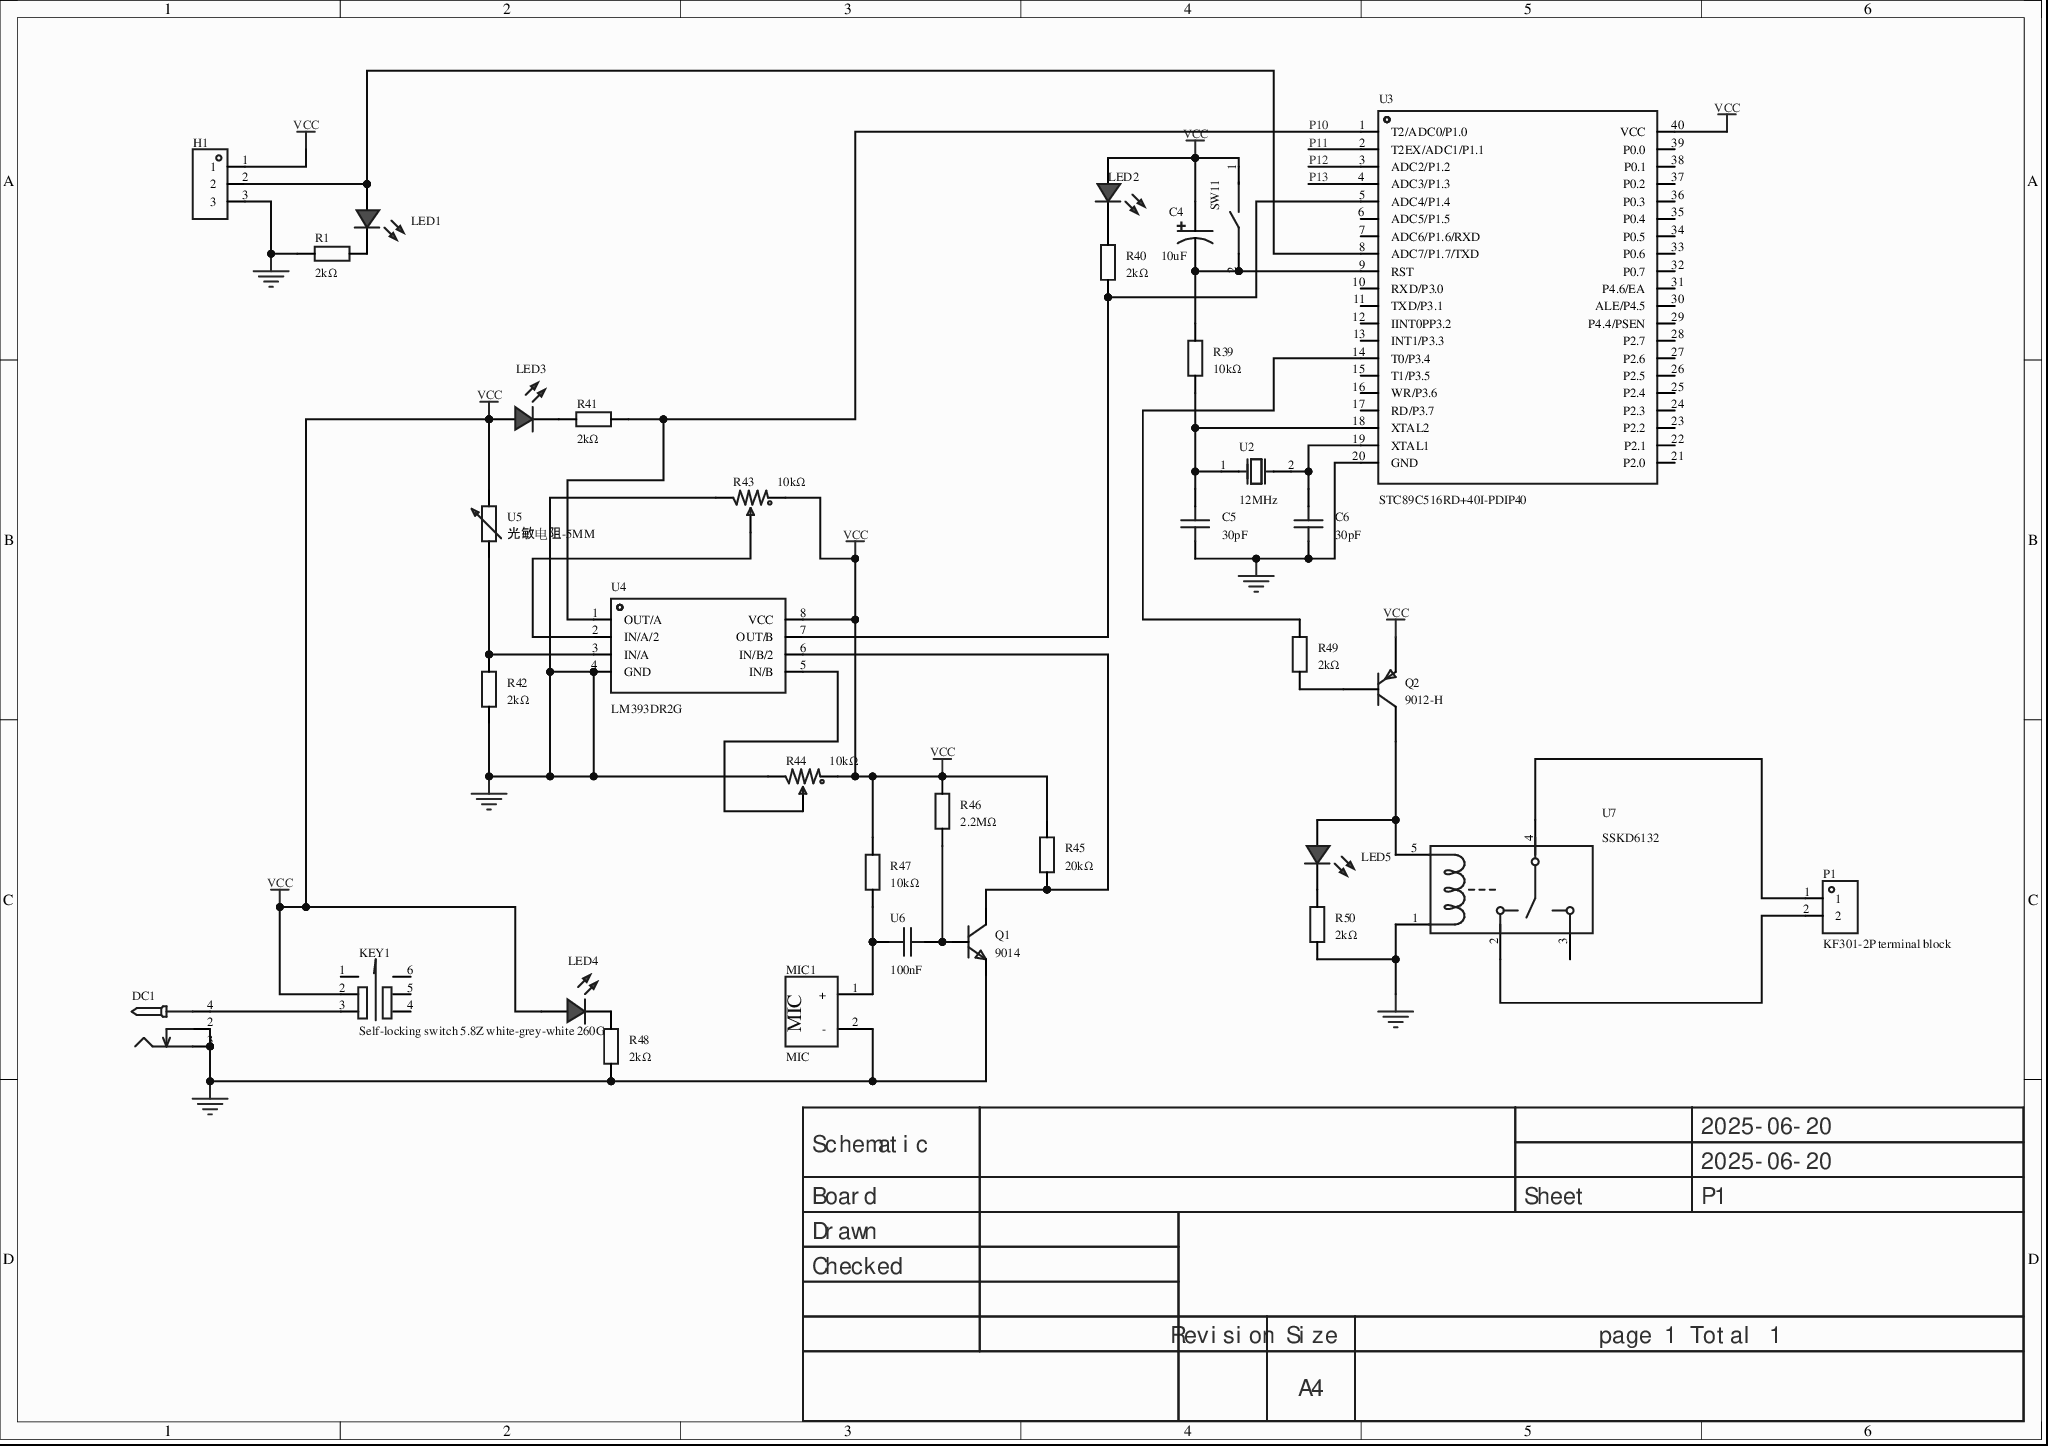
[diagram p0: MISC75177-3.schdoc]
# Altium project MISC75177-2.PrjPcb
1 sheet, 35 parts. Net scope: global (net labels, ports and power ports of the same name join across sheets).
Board file: MISC75177.pcbdoc

## Sheet MISC75177-3.schdoc
size 297 x 209 mm; Version: V1.0; @Project Name: MISC75177; @Page Count: 1; @Update Date: 2025-06-20; @Create Date: 2025-06-20; @Schematic Name: MISC75177; @Page No: 1; @Create Time: 11:09:28; @Update Time: 11:09:28; @Board Name: MISC75177

### Parts
C4  10uF  [CAP-TH_BD6.3-P2.50-D1.0-FD]
C5  30pF  [CAP-TH_L3.6-W2.3-P5.00-D0.5]
C6  30pF  [CAP-TH_L3.6-W2.3-P5.00-D0.5]
DC1  (no value)  [DC-2.0]
H1  (no value)  [HDR-TH_3P-P2.54-V-M]
KEY1  Self-locking switch 5.8Z white-grey-white 260G  [SW-TH_6P-L5.8-W5.8-P2.00-LS4.5-TR]
LED1  (no value)  [LED_TH-3mm]
LED2  (no value)  [LED_TH-3mm]
LED3  (no value)  [LED_TH-3mm]
LED4  (no value)  [LED_TH-3mm]
LED5  (no value)  [LED_TH-3mm]
MIC1  MIC  [MIC-TH_BD6.0-P2.00]
P1  KF301-2P terminal block  [CONN-TH_XY301V-A-5.0-2P]
Q1  9014  [TO-92-3_L4.9-W3.7-P2.54-L]
Q2  9012-H  [TO-92-3_L4.9-W3.7-P1.27-R]
R1  2kΩ  [Res_1/8W]
R39  10kΩ  [Res_1/8W]
R40  2kΩ  [Res_1/8W]
R41  2kΩ  [Res_1/8W]
R42  2kΩ  [Res_1/8W]
R43  10kΩ  [RES-ADJ-SMD_RM065-V1]
R44  10kΩ  [RES-ADJ-SMD_RM065-V1]
R45  20kΩ  [Res_1/8W]
R46  2.2MΩ  [Res_1/8W]
R47  10kΩ  [Res_1/8W]
R48  2kΩ  [Res_1/8W]
R49  2kΩ  [Res_1/8W]
R50  2kΩ  [Res_1/8W]
SW11  Tact switch, 6*6*5 plastic head, 260G, travel 0.25mm, through-hole, middle 2 pins  [KEY-TH_2P-L6.0-W6.0-P5.00]  (value not drawn)
U2  12MHz  [HC-49US_L11.0-W4.6-P4.88]
U3  STC89C516RD+40I-PDIP40  [DIP-40_L52.3-W13.9-P2.54-LS15.2-BL]
U4  LM393DR2G  [SOIC-8_L5.0-W4.0-P1.27-LS6.0-BL]
U5  光敏电阻-5MM  [RES-TH_L4.9-W4.3-P3.4]
U6  100nF  [CAP-TH_L5.0-W2.5-P5.00-D1.0]
U7  SSKD6132  [RELAY-TH_G2R-1]

### Nets
GND: C5.1 C6.1 DC1.2 DC1.3 H1.3 MIC1.2(-) Q1.1(E) R1.1 R42.1 R43.3 R44.3 R48.1 R50.1 U3.20(GND) U4.4(GND) U7.1
VCC: C4.1 H1.1 KEY1.2 LED2.1(C) LED3.1(C) LED4.1(C) Q2.3(E) R43.1 R44.1 R45.2 R46.2 R47.2 SW11.1 U3.40(VCC) U4.8(VCC) U5.2
P10: R41.2 U3.1(T2/ADC0/P1.0) U4.1(OUT/A)
P11: U3.2(T2EX/ADC1/P1.1)
P12: U3.3(ADC2/P1.2)
P13: U3.4(ADC3/P1.3)
NetC4_2: C4.2 R39.2 SW11.2 U3.9(RST)
NetC5_2: C5.2 R39.1 U2.1(OSC1) U3.18(XTAL2)
NetC6_2: C6.2 U2.2(OSC2) U3.19(XTAL1)
NetDC1_4: DC1.4 KEY1.3
NetH1_2: H1.2 LED1.1(C) U3.8(ADC7/P1.7/TXD)
NetLED1_2: LED1.2(A) R1.2
NetLED2_2: LED2.2(A) R40.2
NetLED3_2: LED3.2(A) R41.1
NetLED4_2: LED4.2(A) R48.2
NetLED5_1: LED5.1(C) Q2.1(C) U7.5
NetLED5_2: LED5.2(A) R50.2
NetMIC1_1: MIC1.1(+) R47.1 U6.2
NetP1_1: P1.1 U7.4
NetP1_2: P1.2 U7.2
NetQ1_2: Q1.2(B) R46.1 U6.1
NetQ1_3: Q1.3(C) R45.1 U4.6(IN/B/2)
NetQ2_2: Q2.2(B) R49.1
NetR40_1: R40.1 U3.5(ADC4/P1.4) U4.7(OUT/B)
NetR42_2: R42.2 U4.3(IN/A) U5.1
NetR43_2: R43.2 U4.2(IN/A/2)
NetR44_2: R44.2 U4.5(IN/B)
NetR49_2: R49.2 U3.14(T0/P3.4)

Not connected (* = marked no-connect by the designer): KEY1 1 4 5 6; U3 6(ADC5/P1.5) 7(ADC6/P1.6/RXD) 10(RXD/P3.0) 11(TXD/P3.1) 12(IINT0PP3.2) 13(INT1/P3.3) 15(T1/P3.5) 16(WR/P3.6) 17(RD/P3.7) 21(P2.0) 22(P2.1) 23(P2.2) 24(P2.3) 25(P2.4) 26(P2.5) 27(P2.6) 28(P2.7) 29(P4.4/PSEN) 30(ALE/P4.5) 31(P4.6/EA) 32(P0.7) 33(P0.6) 34(P0.5) 35(P0.4) 36(P0.3) 37(P0.2) 38(P0.1) 39(P0.0); U7 3

### Notes on the sheet
- 2025-06-20
- Schematic
- Board
- Sheet
- P1
- Drawn
- Checked
- Revision
- Size
- A4
- page 1 Total 1

### Library data of the parts
C4 = LKMC1202E100MF: Capacitance: 10uF; tolerance: ±20%; rated voltage: 250V; ripple current: -; equivalent series resistance: -;; Manufacturer: Ymin(永铭); AddInBom: yes; ModelId: 0a4db4bf24b443b3be4905be97ff10c5; ModelTransform: 248.4247,247.99777,0,0,0,0,0,0,-137.795; φD: 6.3mm; L: 12mm; Lifetime @ Temp: 9000hrs@105℃; Symbol: LKMC1202E100MF; Device: LKMC1202E100MF; LCSC Part Name: 10uF ±20% 250V; SupplierPart: C443243; ManufacturerPart: LKMC1202E100MF; Supplier Footprint: 插件,D6.3xL12mm; JLCPCB Part Class: Extended Part; Datasheet: https://example.com/upload/public/pdf/source/20200220/C487520_443A40905984A455D375EE990FEAA9E8.pdf; Supplier: LCSC; ConvertToPcb: yes; FootprintName: CAP-TH_BD6.3-P2.50-D1.0-FD; ModelName: CAP-TH_BD6.3-P2.50-D1.0-FD; Value: 10uF; Tolerance: ±20%; Rated Voltage: 250V; Ripple Current: -; Equivalent Series Resistance(ESR): -; Lead Spacing: 2.5mm
C5 C6 = K300J10C0GF5UH5: Capacitance: 30pF; tolerance: ±5%; rated voltage: 50V; temperature coefficient: C0G;; Manufacturer: VISHAY(威世); AddInBom: yes; ModelId: 8586b865f3f94c6bbd5d7f2c3c951380; ModelName: CAP-TH-2P-L3.6-W2.3-H6.2-P5.0; ModelTransform: 220.472,90.551,0,0,0,0,-0.005,0,-137.795; Symbol: K300J10C0GF5UH5; Device: K300J10C0GF5UH5; LCSC Part Name: 30pF ±5% 50V; SupplierPart: C1623919; ManufacturerPart: K300J10C0GF5UH5; Supplier Footprint: 插件; JLCPCB Part Class: Extended Part; Datasheet: https://example.com/upload/public/pdf/source/20210702/6531D680143ED60327F22057485455BA.pdf; Supplier: LCSC; ConvertToPcb: yes; FootprintName: CAP-TH_L3.6-W2.3-P5.00-D0.5; Value: 30pF; Tolerance: ±5%; Voltage Rated: 50V; Temperature Coefficient: C0G
DC1 = DC-005_2.0: ConvertToPcb: yes; SymbolName: DC power jack; ModelId: f5f20b8a2308479b936ba3c2698865bb0819f05c4eef4c71ace90d822a990e87; ModelName: DC-IN-TH_DC-5520-1; ModelTransform: 372.05,551.18,582.68,90,0,0,137.8,0,-149.61; Device: DC-005_2.0; AddInBom: yes; Supplier Footprint: 插件; FootprintName: DC-2.0
H1 = HDR-M_2.54_1x3P: Symbol: PZ254V-11-03P_C2937625; ConvertToPcb: yes; ModelId: bb473b6d38ff42a99216a4fcdbdcc4cb; ModelName: HDR-TH_3P-P2.54-M-LI-1X3P; ModelTransform: 299.9994,100,0,0,0,0,0,0,-118.11; Device: HDR-M_2.54_1x3P; AddInBom: yes; SupplierPart: C2937625; Supplier Footprint: 插件; FootprintName: HDR-TH_3P-P2.54-V-M
KEY1 = 自锁开关 5.8Z白灰白260G: Heat resistance 260 degrees; Symbol: Self-locking switch 5.8ZWhite and white260G; AddInBom: yes; ModelId: cd839ddf8c8d4e01911ba601e759d3e9; ModelTransform: 228.346,228.346,0,0,0,0,0,0,-137.795; Device: Self-locking switch 5.8Z white-grey-white 260G; LCSC Part Name: 自锁开关 5.8Z白灰白 260G  5.8*5.8mm; SupplierPart: C56857; ManufacturerPart: 自锁开关 5.8Z白灰白260G; Supplier Footprint: 插件; JLCPCB Part Class: Extended Part; Supplier: LCSC; ConvertToPcb: yes; FootprintName: SW-TH_6P-L5.8-W5.8-P2.00-LS4.5-TR; ModelName: SW-TH_6P-L5.8-W5.8-P2.00-LS4.5-TR
LED1-LED5 = LED_TH-R_3mm: ConvertToPcb: yes; ModelId: a497c992633541038a38947cdc58012f; ModelName: LED-TH-3mm_R; ModelTransform: 141.274,153.327,0,0,0,0,-5.984,0,-137.795; Symbol: LED_TH-R; Device: LED_TH-R_3mm; AddInBom: yes; FootprintName: LED_TH-3mm; Supplier Footprint: 插件
MIC1 = MIC: Symbol: MIC_C9900023869; AddInBom: yes; ModelId: 3d52db69e70846c48297d60920796834; ModelTransform: 228.346,228.21852,0,0,0,0,0,0,-78.74; Device: MIC; LCSC Part Name: MIC; SupplierPart: C9900023869; ManufacturerPart: MIC; Supplier Footprint: THrough hole; Supplier: LCSC; ConvertToPcb: yes; FootprintName: MIC-TH_BD6.0-P2.00; ModelName: MIC-TH_BD6.0-P2.00
P1 = KF301-2P接线端子: AddInBom: yes; ModelId: ef7ead88b0f2448d904975b26718870f; ModelTransform: 417.322,299.212,0,0,0,0,11.811,-7.835,-157.48; Symbol: KF301-2P terminal block; Device: KF301-2P terminal block; LCSC Part Name: KF301-2P接线端子; SupplierPart: C9900016950; ManufacturerPart: KF301-2P接线端子; Supplier Footprint: CK301-2P; JLCPCB Part Class: Extended Part; Supplier: LCSC; ConvertToPcb: yes; FootprintName: CONN-TH_XY301V-A-5.0-2P; ModelName: CONN-TH_XY301V-A-5.0-2P
Q1 = 9014: Transistor type: NPN; collector current (Ic): 100mA; collector-emitter breakdown voltage (Vceo): 45V; power dissipation (Pd): 450mW;; Manufacturer: BLUE ROCKET(蓝箭); AddInBom: yes; ModelId: ff77d7980f5c4c0980cec2e309db67c4; ModelTransform: 222.047,139.764,0,180,0,0,0,28.661,-196.85; Current - Collector Cutoff: 50nA; Symbol: 9014; Device: 9014; LCSC Part Name: 9014; SupplierPart: C3037604; ManufacturerPart: 9014; Supplier Footprint: TO-92-2.54mm; Supplier: LCSC; ConvertToPcb: yes; FootprintName: TO-92-3_L4.9-W3.7-P2.54-L; ModelName: TO-92-3_L4.9-W3.7-P2.54-L; type: NPN; Current - Collector(Ic): 100mA; Collector - Emitter Voltage VCEO: 45V; Pd - Power Dissipation: 450mW
Q2 = 9012-H: Transistor type: PNP; collector current (Ic): 500mA; collector-emitter breakdown voltage (Vceo): 20V; power dissipation (Pd): 625mW; DC current gain (hFE): 144@50mA,1V;; Manufacturer: BLUE ROCKET(蓝箭); AddInBom: yes; ModelId: fb6e5510710348aa920d5dcb21565449; ModelName: TO-92-3_L4.9-W3.7-H5.3-P1.27-R; ModelTransform: 176.28752,144.88554,0,180,0,0,0,20.512,-196.85; Current - Collector Cutoff: 100nA; Vce Saturation(VCE(sat)): 180mV; Symbol: 9012-H; Device: 9012-H; LCSC Part Name: 9012-H; SupplierPart: C305407; ManufacturerPart: 9012-H; Supplier Footprint: TO-92-3; JLCPCB Part Class: Extended Part; Datasheet: https://example.com/upload/public/pdf/source/20181016/C305407_783ADA743A5C7538C7EEEE88BE9BF32D.pdf; Supplier: LCSC; ConvertToPcb: yes; FootprintName: TO-92-3_L4.9-W3.7-P1.27-R; type: PNP; Current - Collector(Ic): 500mA; Collector - Emitter Voltage VCEO: 20V; Pd - Power Dissipation: 625mW; DC Current Gain: 144@50mA,1V; Transition frequency(fT): -; Operating Temperature: -
R1 R40-R42 R45-R50 = Res_AXIAL-1/8W: ConvertToPcb: yes; SymbolName: Resistor; ModelId: b2b5ae7ae4c642178fe0039925c86a3f; ModelName: RES-TH_BD1.8-L3.2-P7.20-D0.4; ModelTransform: 282.86,66.88,253.09,0,0,0,0,0,-191; Device: Res_AXIAL-1/8W; AddInBom: yes; Supplier Footprint: 轴向引线; FootprintName: Res_1/8W
  R1 R40-R42 R48-R50: Value: 2kΩ
  R45: Value: 20kΩ
  R46: Value: 2.2MΩ
  R47: Value: 10kΩ
R39 = Res_AXIAL-1/8W: Symbol: Resistor; ConvertToPcb: yes; ModelId: b2b5ae7ae4c642178fe0039925c86a3f; ModelName: RES-TH_BD1.8-L3.2-P7.20-D0.4; ModelTransform: 282.86,66.88,253.09,0,0,0,0,0,-191; Device: Res_AXIAL-1/8W; AddInBom: yes; Supplier Footprint: 轴向引线; Value: 10kΩ; FootprintName: Res_1/8W
R43 R44 = RM065-103(10K): Resistance: 10kΩ; tolerance: ±25%; power: 100mW;; Manufacturer: BOCHEN(博晨); AddInBom: yes; ModelId: c816c2b7942147f5a832150e8ef6960c; ModelTransform: 255.905,283.464,0,0,0,0,0.025,-3.937,-157.48; Symbol: RM065-103(10K); Device: RM065-103(10K); LCSC Part Name: 10kΩ ±25%; SupplierPart: C5205021; ManufacturerPart: RM065-103(10K); Supplier Footprint: 插件; JLCPCB Part Class: Extended Part; Datasheet: https://example.com/upload/public/pdf/source/20221019/6263C46FBC7F1B66CBAADA74DC5EFAA2.pdf; Supplier: LCSC; ConvertToPcb: yes; FootprintName: RES-ADJ-SMD_RM065-V1; ModelName: RES-ADJ-SMD_RM065-V1; Value: 10kΩ; Tolerance: ±25%; Power(Watts): 100mW
SW11 = 轻触开关,6*6*5塑头,260G,行程0.25mm,直插中2脚: Symbol: SWITCH,6*6*5PLASTIC HEAD,260G, 0.25MM,DIP2; AddInBom: yes; ModelId: d13ad252cbf84dc495704a853cd2bab6; ModelName: KEY-TH_2P-L6.0-W6.0-H5.0-P5.00; ModelTransform: 236.22,236.22,0,0,0,0,0,0,-137.795; Device: Tact switch, 6*6*5 plastic head, 260G, travel 0.25mm, through-hole, middle 2 pins; LCSC Part Name: 轻触开关,6*6*5塑头,260G,行程0.25mm,直插中2脚; SupplierPart: C71845; ManufacturerPart: 轻触开关,6*6*5塑头,260G,行程0.25mm,直插中2脚; Supplier Footprint: 插件; JLCPCB Part Class: Extended Part; Supplier: LCSC; ConvertToPcb: yes; FootprintName: KEY-TH_2P-L6.0-W6.0-P5.00
U2 = ECS-120-S-4: Frequency: 12MHz; room-temperature frequency tolerance: ±30ppm; external load capacitance: -; frequency stability (full temperature): ±50ppm;; Manufacturer: ECS; AddInBom: yes; ModelId: 59d05c800eee432cb051aa4925461fda; ModelName: HC-49US_L11.0-W4.7-H3.5-P4.88; ModelTransform: 432.44473,183.0705,0,0,0,0,0,0,-137.795; Equivalent Series Resistance (ESR): 60Ω; Symbol: ECS-120-S-4; Device: ECS-120-S-4; LCSC Part Name: 12MHz ±30ppm; ManufacturerPart: ECS-120-S-4; Supplier Footprint: HC-49S; JLCPCB Part Class: Extended Part; Datasheet: https://example.com/upload/public/pdf/source/20210402/81F084B668D60DFAE850A61100CCABAF.pdf; Supplier: LCSC; ConvertToPcb: yes; FootprintName: HC-49US_L11.0-W4.6-P4.88; Value: 12MHz; Normal temperature Frequency Tolerance: ±30ppm; External load capacitor: -; Frequency Stability(Full temperature range): ±50ppm; Operating Temperature: -10℃~+70℃
U3 = STC89C516RD+40I-PDIP40: CPU core: 51 series; program memory capacity: 61KB; total RAM: 1.25KB; GPIO port count: 35; operating voltage range: 3.5V~5.5V; max CPU frequency: -; program memory type: FLASH;; Manufacturer: STC(宏晶); AddInBom: yes; ModelId: 16d4686a009b4ddca948f91eddb57b14; ModelName: DIP-40_L52.3-W13.8-H4.0-LS15.24-P2.54; ModelTransform: 2059.051,615.743,0,0,0,0,0,0,-129.921; GPIO Ports Number: 35; 16Bit Timer: 3; UART/USART: 1; Peripheral/Function: Watchdog; Symbol: STC89C516RD+40I-PDIP40; Device: STC89C516RD+40I-PDIP40; LCSC Part Name: STC89C516RD+40I-PDIP40; SupplierPart: C52225; ManufacturerPart: STC89C516RD+40I-PDIP40; Supplier Footprint: DIP-40; JLCPCB Part Class: Extended Part; Datasheet: https://example.com/upload/public/pdf/source/20180614/C87831_BBAF7FB8B286C29ACE4E9B180C033FEC.pdf; Supplier: LCSC; ConvertToPcb: yes; FootprintName: DIP-40_L52.3-W13.9-P2.54-LS15.2-BL; CPU Core: 51 series; Program Storage Size: 61KB; RAM Size: 1.25KB; Operating Voltage Range: 3.5V~5.5V; CPU Maximum Speed: -; Program Memory Type: FLASH; Operating Temperature Range: -40℃~+85℃; ADC (Bit): -; DAC (Bit): -; PWM (Bit): -; 8Bit Timer: -; 32Bit Timer: -; CAN: -; I2C: -; I2S: -; SPI: -; Universal Serial Bus: -; Internal Comparator: -; communication protocol: -; Watchdog: Yes; Real-Time Clock: -; Infrared Data Association: -; Low-Voltage Detect: -; CCP Capture/Compare: -; Secure Digital Input and Output: -; Direct Memory Access: -; Internal Oscillator: -
U4 = LM393DR2G: Comparators: dual; input offset voltage (Vos): 5mV; input bias current (Ib): 25nA;; Manufacturer: onsemi(安森美); AddInBom: yes; ModelId: e81d2f7d937b4a6ab1dca543ff5d56a4; ModelName: SOIC-8_L4.9-W3.9-H1.7-LS6.0-P1.27; ModelTransform: 189.751,236.22,0,0,0,0,-0.0005,0.0005,0; Propagation Delay Time: 300ns; Voltage - Supply: 2V~36V; Output Type: TTL; CMOS; Quiescent Current per Amplifier: 400uA; Symbol: LM393DR2G; Device: LM393DR2G; LCSC Part Name: LM393DR2G; SupplierPart: C7955; ManufacturerPart: LM393DR2G; Supplier Footprint: SOIC-8; JLCPCB Part Class: Basic Part; Datasheet: https://example.com/upload/public/pdf/source/20140815/1457707223499.pdf; Supplier: LCSC; ConvertToPcb: yes; FootprintName: SOIC-8_L5.0-W4.0-P1.27-LS6.0-BL; Number of Channels: Dual; Vos - Input Offset Voltage: 5mV; Ib - Input Bias Current: 25nA; Input Hysteresis Voltage (Vhys): -; Common Mode Rejection Ratio(CMRR): -; Operating Temperature: -40℃~+125℃
U5 = 光敏电阻-5MM: AddInBom: yes; ModelId: 8cda4899688949e78503a56fe341541c; ModelTransform: 169.291,200.6107,0,90,0,0,0,0,-196.85; Symbol: 光敏电阻-5MM; Device: 光敏电阻-5MM; LCSC Part Name: 光敏电阻-5MM; SupplierPart: C9900003115; ManufacturerPart: 光敏电阻-5MM; Supplier Footprint: RES-TH_4.3X4.9X3.37P; JLCPCB Part Class: Extended Part; Supplier: LCSC; ConvertToPcb: yes; FootprintName: RES-TH_L4.9-W4.3-P3.4; ModelName: RES-TH_L4.9-W4.3-P3.4
U6 = 100nF: Symbol: 100NF_C9900015256; AddInBom: yes; ModelId: 08e3d7481fc7486bb1b263873f51e1e1; ModelName: CAP-TH_BD5.0-W2.5-P5.08; ModelTransform: 224.652,98.425,0,0,0,0,-0.005,0,-137.795; Device: 100nF; LCSC Part Name: 100nF; SupplierPart: C9900015256; ManufacturerPart: 100nF; Supplier Footprint: CAP-TH_L5.0-W2.5-P5.00-D1.0; Supplier: LCSC; ConvertToPcb: yes; FootprintName: CAP-TH_L5.0-W2.5-P5.00-D1.0
U7 = SSKD6132: AddInBom: yes; ModelId: fe99462dd15043c98af5adb0e5338dda; ModelTransform: 1141.73,511.81,0,0,0,0,26.417,-0.354,-157.48; Symbol: SSKD6132; Device: SSKD6132; LCSC Part Name: SSKD6132; SupplierPart: C9900012103; ManufacturerPart: SSKD6132; Supplier Footprint: RELAY-TH_G2R-1; JLCPCB Part Class: Extended Part; Supplier: LCSC; ConvertToPcb: yes; FootprintName: RELAY-TH_G2R-1; ModelName: RELAY-TH_G2R-1